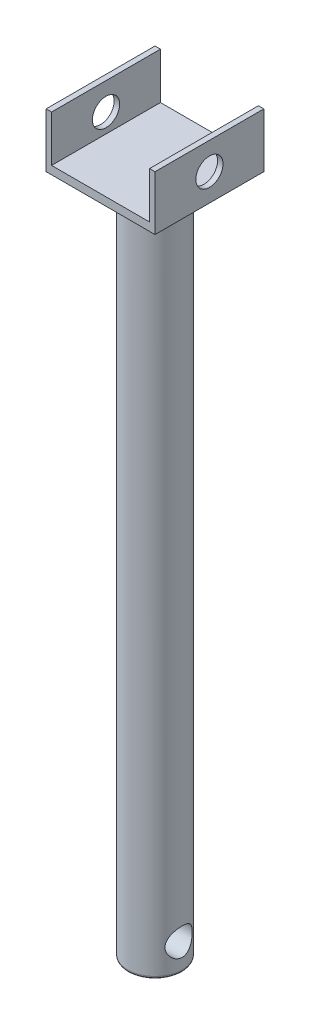
from build123d import *

# Parameters (mm, degrees)
BOSS_EXTRUDE1_DEPTH     = 400
SKETCH2_R               = 50
CUT_EXTRUDE1_DEPTH      = 400
SKETCH3_R               = 100
BOSS_EXTRUDE2_DEPTH     = 2500
CUT_EXTRUDE2_DEPTH      = 2500
CUT_EXTRUDE2_DEPTH_BACK = 2500
SKETCH4_R               = 50
FILLET1_R               = 10


with BuildPart() as part:
    # Sketch1 → Boss-Extrude1 (new body)
    with BuildSketch(Plane.XY):
        Polygon((-180, 0), (180, 0), (180, 170), (200, 170), (200, -30), (-200, -30), (-200, 170), (-180, 170), align=None)
    extrude(amount=BOSS_EXTRUDE1_DEPTH)

    # Sketch2 → Cut-Extrude1 (cut)
    with BuildSketch(Plane(origin=(200, 0, 0), x_dir=(0, 0, -1), z_dir=(1, 0, 0))):
        with Locations(Location((-200, 70, 0), (0, 0, 90))):
            Circle(SKETCH2_R)
    extrude(amount=-CUT_EXTRUDE1_DEPTH, mode=Mode.SUBTRACT)

    # Sketch3 → Boss-Extrude2 (add)
    with BuildSketch(Plane.XZ.offset(30)):
        with Locations(Location((0, 200, 0), (0, 0, 180))):
            Circle(SKETCH3_R)
    extrude(amount=BOSS_EXTRUDE2_DEPTH)

    # Sketch4 → Cut-Extrude2 (cut, two sides: drawn at the far end of the back side and taken through both)
    with BuildSketch(Plane(origin=(0, 0, 0), x_dir=(0, 0, -1), z_dir=(1, 0, 0)).offset(-CUT_EXTRUDE2_DEPTH_BACK)):
        with Locations(Location((-200, -2430, 0), (0, 0, 180))):
            Circle(SKETCH4_R)
    extrude(amount=CUT_EXTRUDE2_DEPTH + CUT_EXTRUDE2_DEPTH_BACK, mode=Mode.SUBTRACT)

    # Fillet1
    fillet1_edges = [part.edges().sort_by_distance(p)[0] for p in [
        (100, -2530, 200),
    ]]
    fillet(fillet1_edges, radius=FILLET1_R)


solid = part.part
